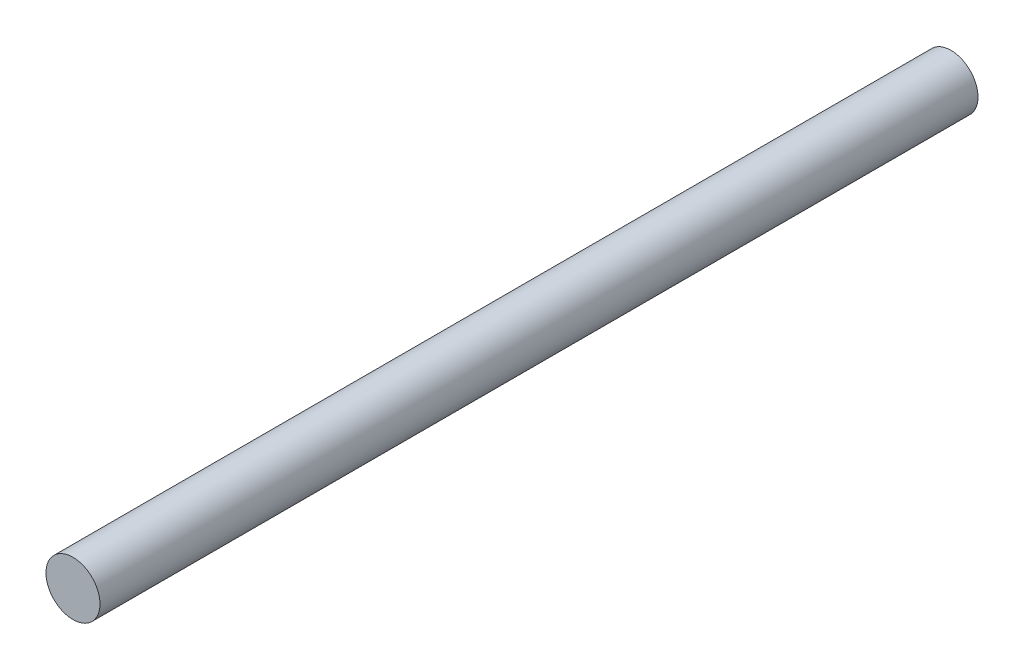
from build123d import *

# Parameters (mm, degrees)
SKETCH1_R           = 4
BOSS_EXTRUDE1_DEPTH = 130


with BuildPart() as part:
    # Sketch1 → Boss-Extrude1 (new body)
    with BuildSketch(Plane.XY):
        with Locations((233.370511684, 361.800592491)):
            Circle(SKETCH1_R)
    extrude(amount=-BOSS_EXTRUDE1_DEPTH)


solid = part.part
